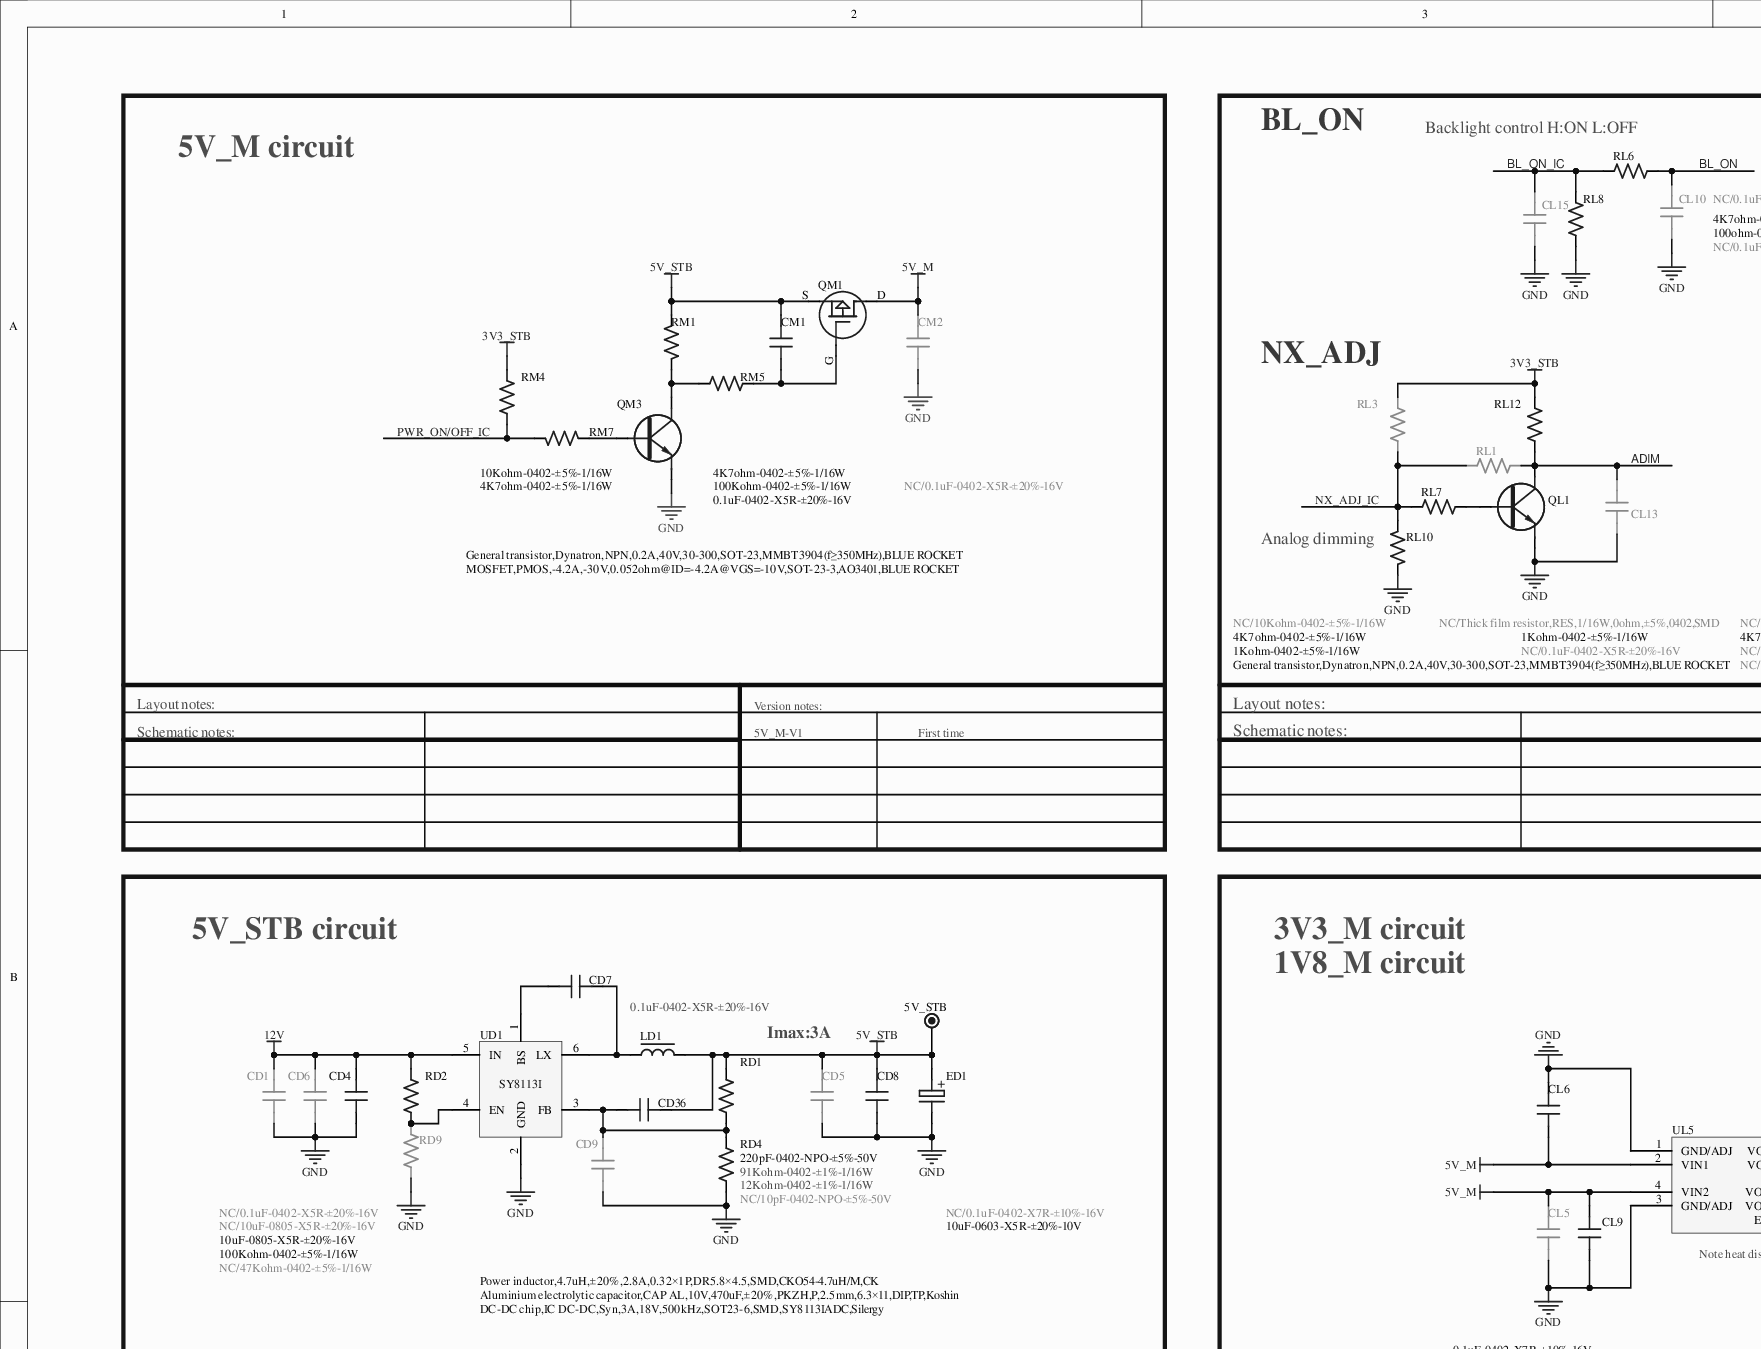
[diagram p0: MISC84395-7.SchDoc, top left]
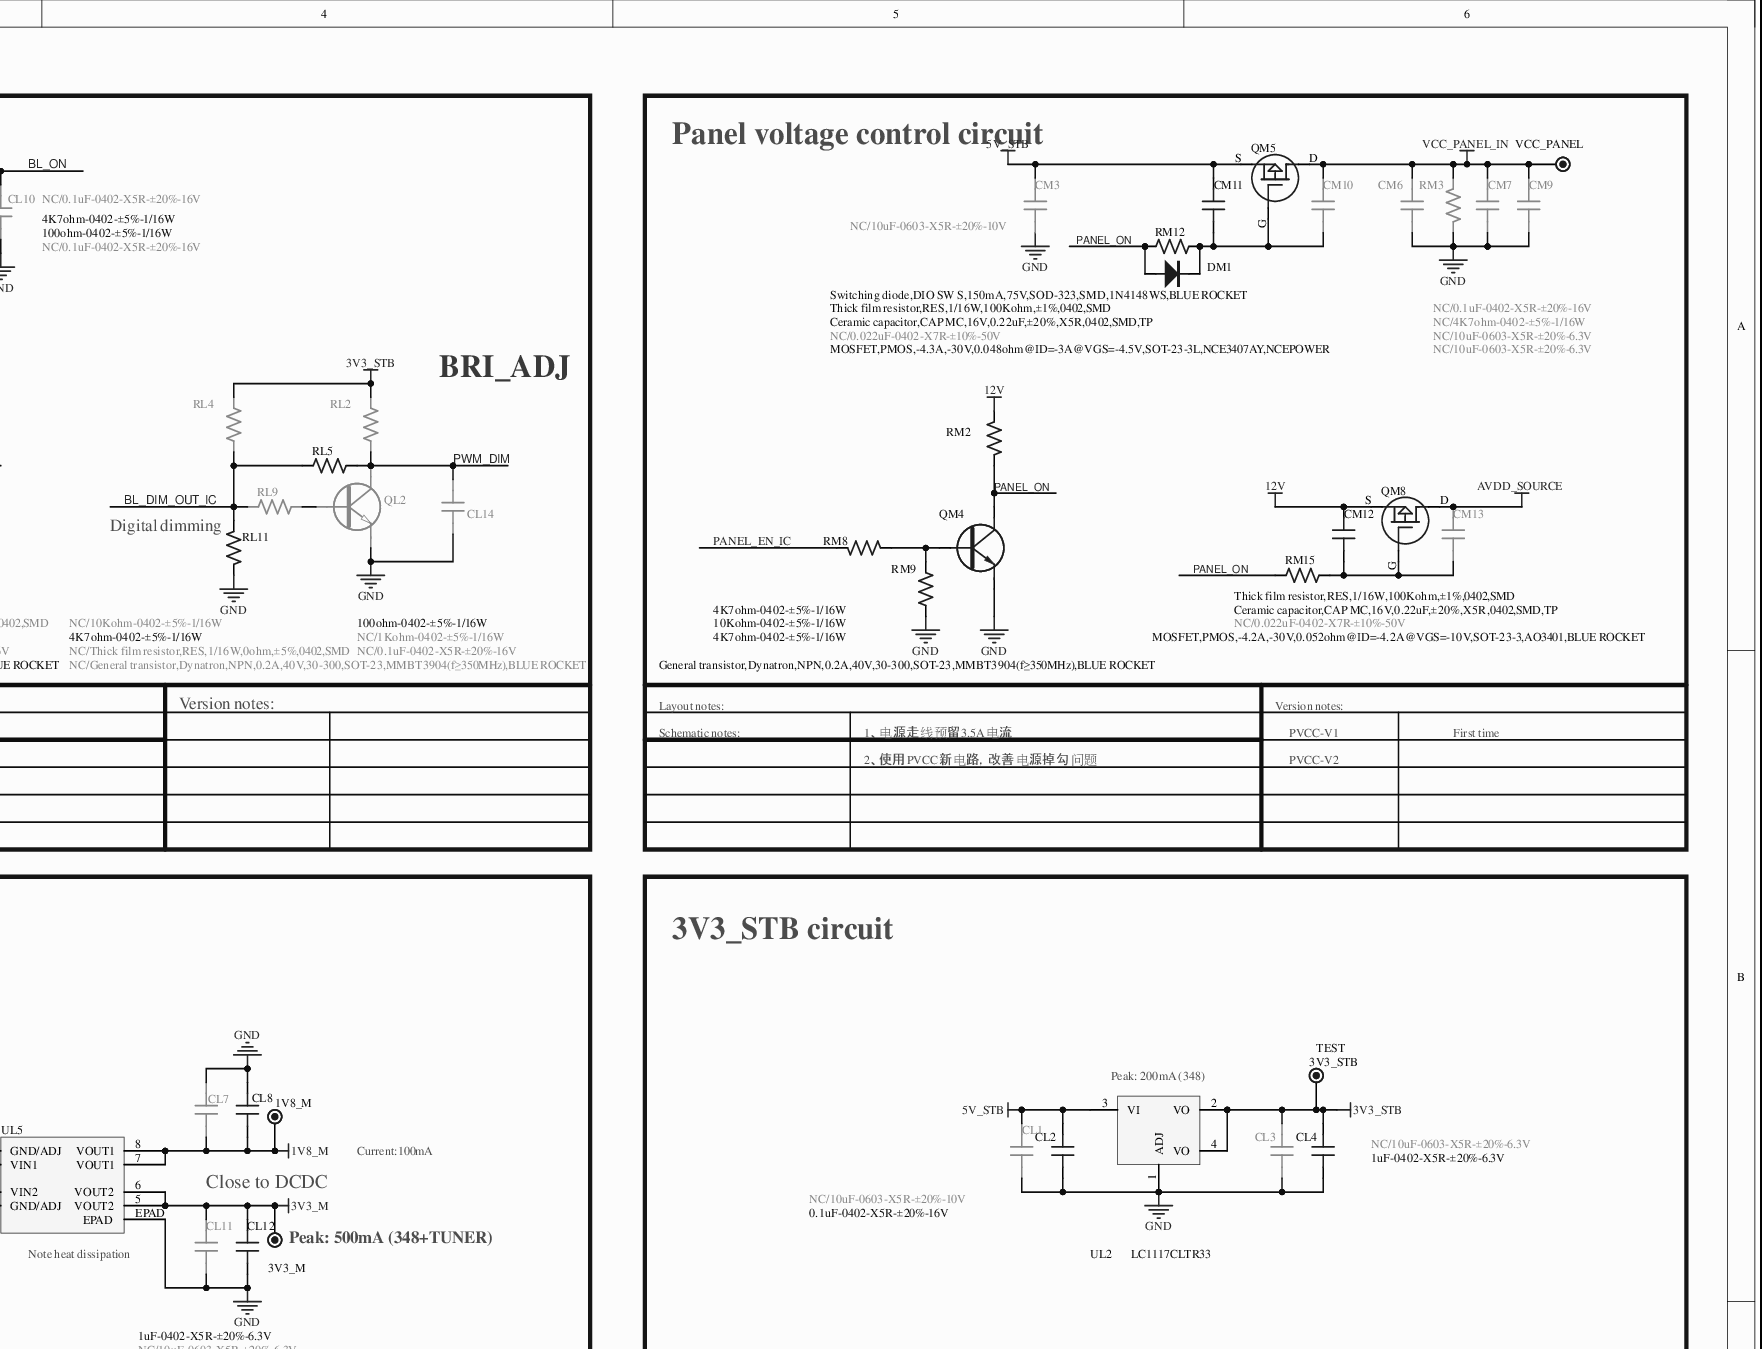
[diagram p1: MISC84395-7.SchDoc, top right]
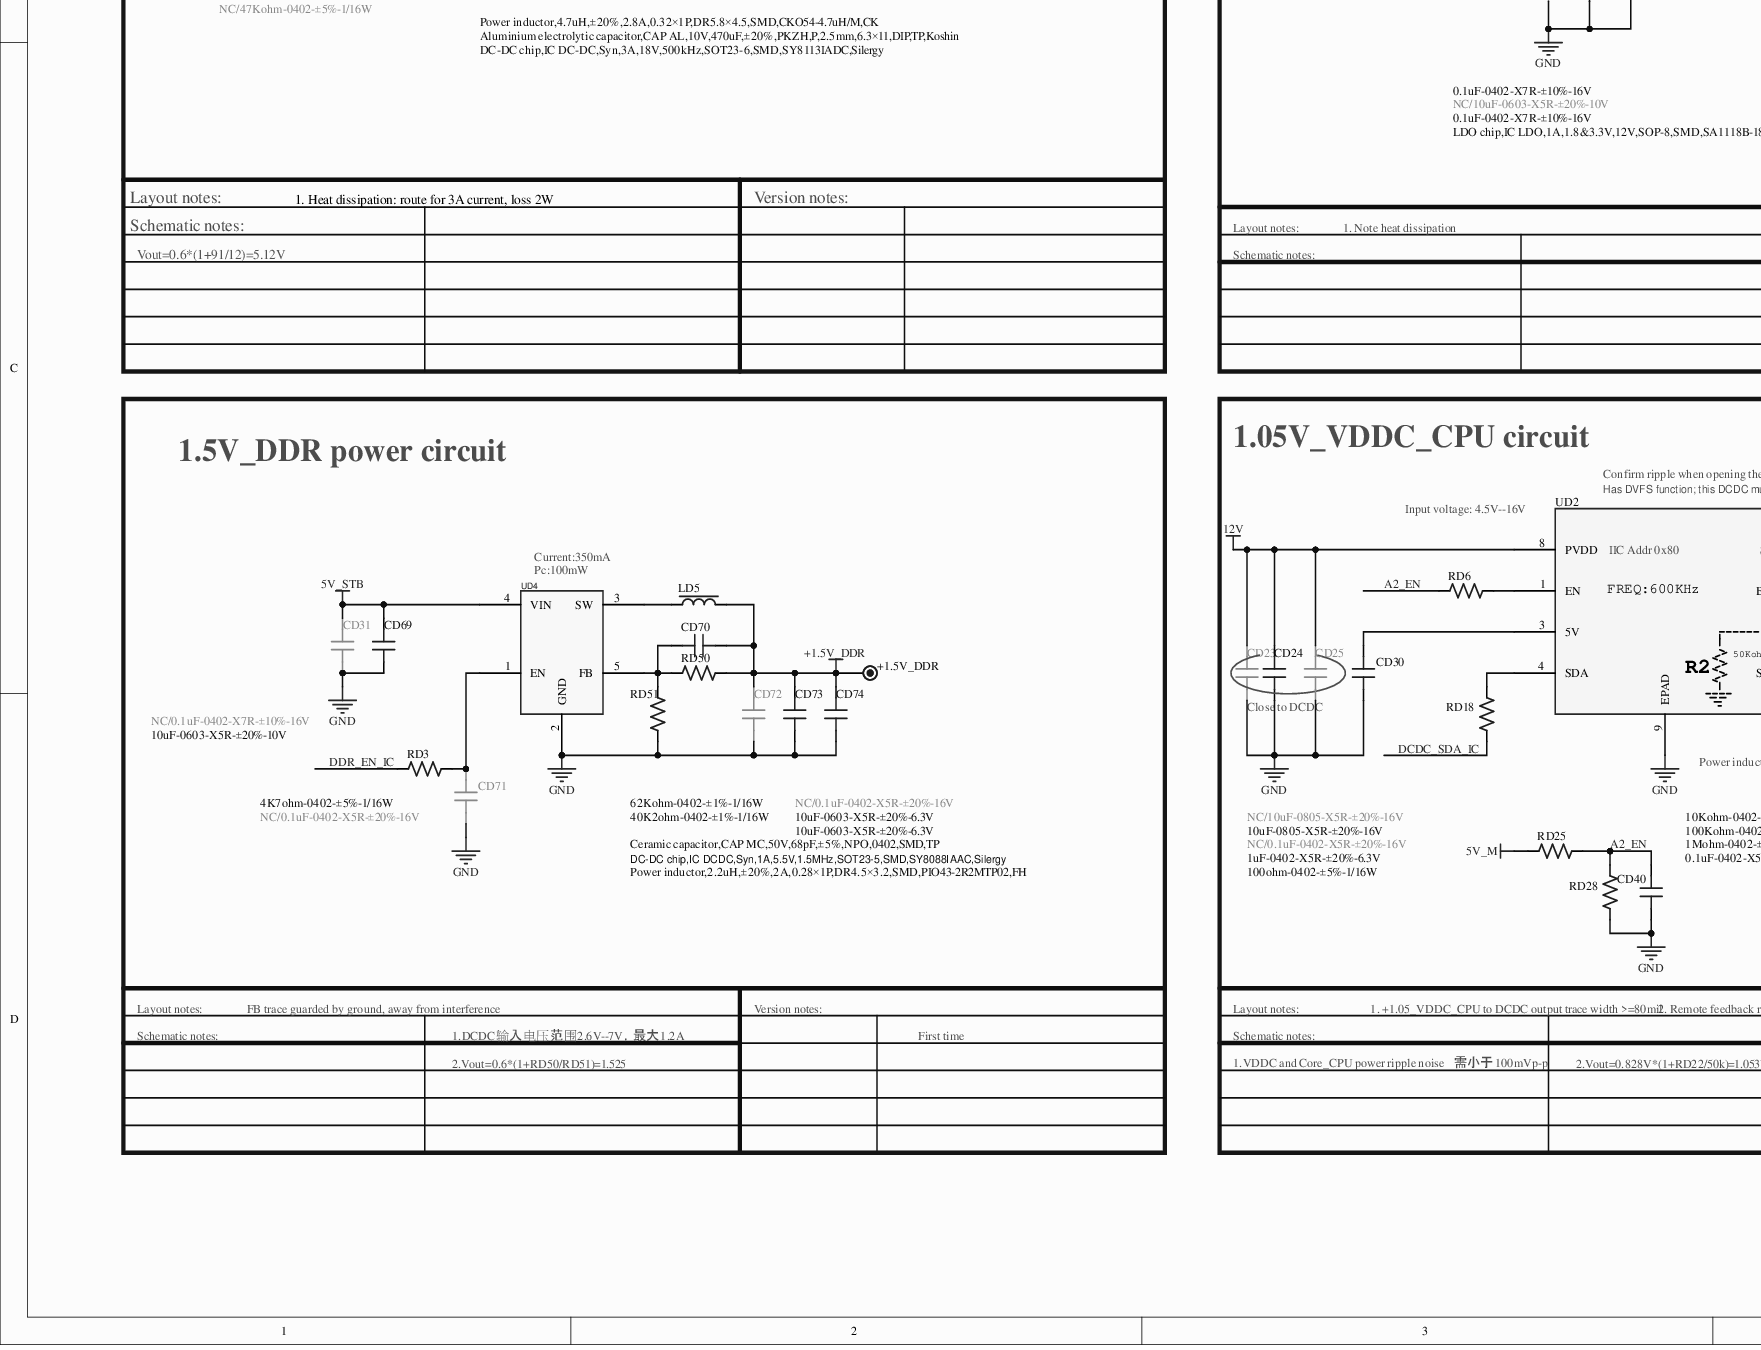
[diagram p2: MISC84395-7.SchDoc, bottom left]
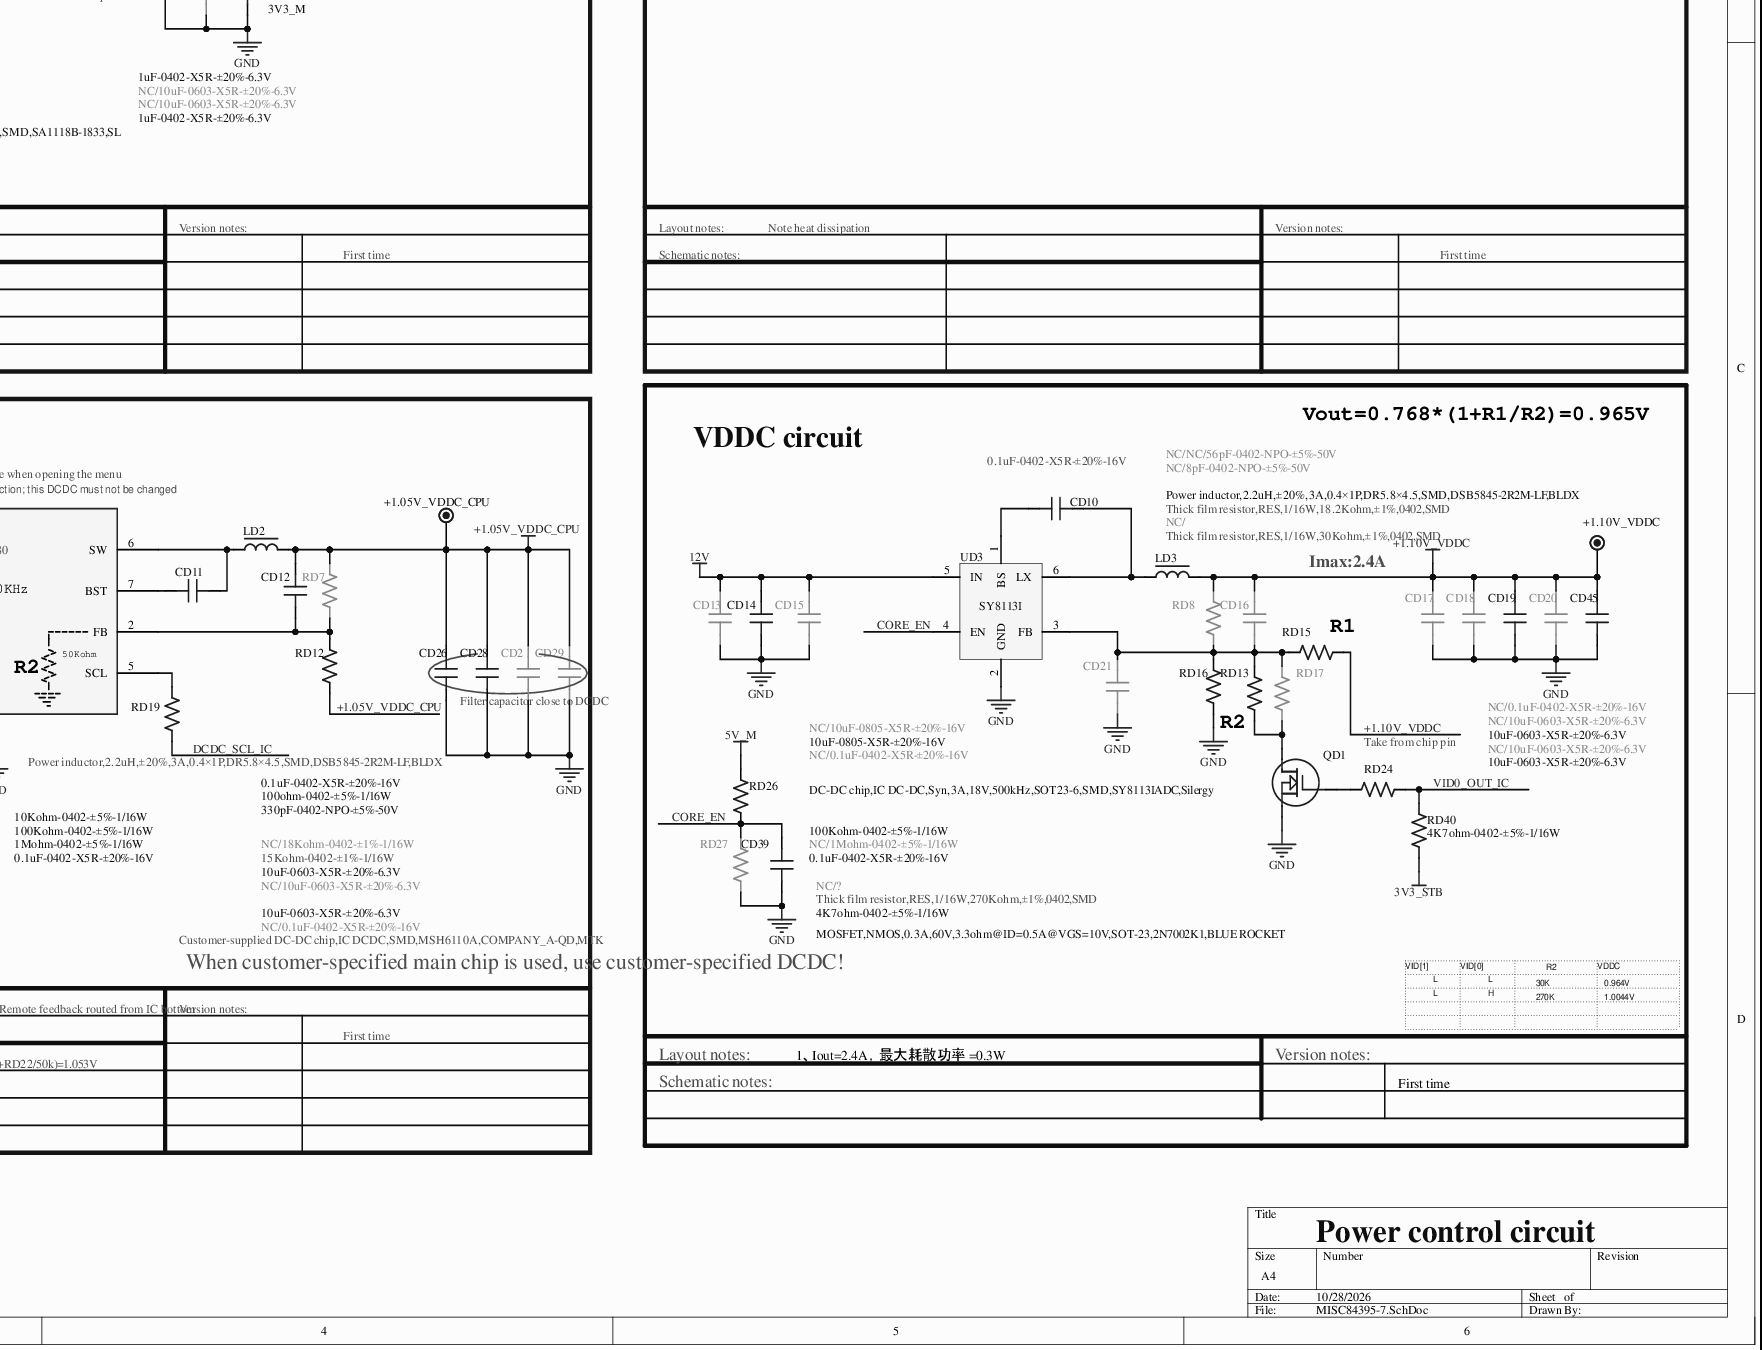
[diagram p3: MISC84395-7.SchDoc, bottom right]
# Altium project MISC84395-37.PrjPCB (part 4 of 13)

## Sheet MISC84395-7.SchDoc
size 635 x 482 mm

### Parts
1V8_M  TEST  [TP]  (value not drawn)
3V3_M  TEST  [TP]  (value not drawn)
3V3_STB  TEST  [TP]
5V_STB  TEST  [TP]  (value not drawn)
+1.5V_DDR  TEST  [TP]  (value not drawn)
+1.05V_VDDC_CPU  TEST  [TP]  (value not drawn)
+1.10V_VDDC  TEST  [TP]  (value not drawn)
CD1  NC/0.1uF-0402-X5R-±20%-16V  [C0402]
CD2  NC/10uF-0603-X5R-±20%-6.3V  [C0603]
CD4  10uF-0805-X5R-±20%-16V  [C0805]
CD5  NC/0.1uF-0402-X7R-±10%-16V  [C0402]
CD6  NC/10uF-0805-X5R-±20%-16V  [C0805]
CD7  0.1uF-0402-X5R-±20%-16V  [C0402]
CD8  10uF-0603-X5R-±20%-10V  [C0603]
CD9  NC/10pF-0402-NPO-±5%-50V  [C0402]
CD10  0.1uF-0402-X5R-±20%-16V  [C0402]
CD11  0.1uF-0402-X5R-±20%-16V  [C0402]
CD12  330pF-0402-NPO-±5%-50V  [C0402]
CD13  NC/10uF-0805-X5R-±20%-16V  [C0805]
CD14  10uF-0805-X5R-±20%-16V  [C0805]
CD15  NC/0.1uF-0402-X5R-±20%-16V  [C0402]
CD16  NC/NC/56pF-0402-NPO-±5%-50V  [C0402]
CD17  NC/0.1uF-0402-X5R-±20%-16V  [C0402]
CD18  NC/10uF-0603-X5R-±20%-6.3V  [C0603]
CD19  10uF-0603-X5R-±20%-6.3V  [C0603]
CD20  NC/10uF-0603-X5R-±20%-6.3V  [C0603]
CD21  NC/8pF-0402-NPO-±5%-50V  [C0402]
CD23  NC/10uF-0805-X5R-±20%-16V  [C0805]
CD24  10uF-0805-X5R-±20%-16V  [C0805]
CD25  NC/0.1uF-0402-X5R-±20%-16V  [C0402]
CD26  10uF-0603-X5R-±20%-6.3V  [C0603]
CD28  10uF-0603-X5R-±20%-6.3V  [C0603]
CD29  NC/0.1uF-0402-X5R-±20%-16V  [C0402]
CD30  1uF-0402-X5R-±20%-6.3V  [C0402]
CD31  NC/0.1uF-0402-X7R-±10%-16V  [C0402]
CD36  220pF-0402-NPO-±5%-50V  [C0402]
CD39  0.1uF-0402-X5R-±20%-16V  [C0402]
CD40  0.1uF-0402-X5R-±20%-16V  [C0402]
CD45  10uF-0603-X5R-±20%-6.3V  [C0603]
CD69  10uF-0603-X5R-±20%-10V  [C0603]
CD70  Ceramic capacitor,CAP MC,50V,68pF,±5%,NPO,0402,SMD,TP  [C0402]
CD71  NC/0.1uF-0402-X5R-±20%-16V  [C0402]
CD72  NC/0.1uF-0402-X5R-±20%-16V  [C0402]
CD73  10uF-0603-X5R-±20%-6.3V  [C0603]
CD74  10uF-0603-X5R-±20%-6.3V  [C0603]
CL1  NC/10uF-0603-X5R-±20%-10V  [C0603]
CL2  0.1uF-0402-X5R-±20%-16V  [C0402]
CL3  NC/10uF-0603-X5R-±20%-6.3V  [C0603]
CL4  1uF-0402-X5R-±20%-6.3V  [C0402]
CL5  NC/10uF-0603-X5R-±20%-10V  [C0603]
CL6  0.1uF-0402-X7R-±10%-16V  [C0402]
CL7  NC/10uF-0603-X5R-±20%-6.3V  [C0603]
CL8  1uF-0402-X5R-±20%-6.3V  [C0402]
CL9  0.1uF-0402-X7R-±10%-16V  [C0402]
CL10  NC/0.1uF-0402-X5R-±20%-16V  [C0402]
CL11  NC/10uF-0603-X5R-±20%-6.3V  [C0603]
CL12  1uF-0402-X5R-±20%-6.3V  [C0402]
CL13  NC/0.1uF-0402-X5R-±20%-16V  [C0402]
CL14  NC/0.1uF-0402-X5R-±20%-16V  [C0402]
CL15  NC/0.1uF-0402-X5R-±20%-16V  [C0402]
CM1  0.1uF-0402-X5R-±20%-16V  [C0402]
CM2  NC/0.1uF-0402-X5R-±20%-16V  [C0402]
CM3  NC/10uF-0603-X5R-±20%-10V  [C0603]
CM6  NC/0.1uF-0402-X5R-±20%-16V  [C0402]
CM7  NC/10uF-0603-X5R-±20%-6.3V  [C0603]
CM9  NC/10uF-0603-X5R-±20%-6.3V  [C0603]
CM10  NC/0.022uF-0402-X7R-±10%-50V  [C0402]
CM11  Ceramic capacitor,CAP MC,16V,0.22uF,±20%,X5R,0402,SMD,TP  [C0402]
CM12  Ceramic capacitor,CAP MC,16V,0.22uF,±20%,X5R,0402,SMD,TP  [C0402]
CM13  NC/0.022uF-0402-X7R-±10%-50V  [C0402]
DM1  Switching diode,DIO SW S,150mA,75V,SOD-323,SMD,1N4148WS,BLUE ROCKET  [DIODE-S-12]
ED1  Aluminium electrolytic capacitor,CAP AL,10V,470uF,±20%,PKZH,P,2.5mm,6.3×11,DIP,TP,Koshin  [EC(6.3*11)-V-2.5]
LD1  Power inductor,4.7uH,±20%,2.8A,0.32×1P,DR5.8×4.5,SMD,CKO54-4.7uH/M,CK  [L(6.0*4.5)-S]
LD2  Power inductor,2.2uH,±20%,3A,0.4×1P,DR5.8×4.5,SMD,DSB5845-2R2M-LF,BLDX  [L(5.8*4.5)-S]
LD3  Power inductor,2.2uH,±20%,3A,0.4×1P,DR5.8×4.5,SMD,DSB5845-2R2M-LF,BLDX  [L(5.8*4.5)-S]
LD5  Power inductor,2.2uH,±20%,2A,0.28×1P,DR4.5×3.2,SMD,PIO43-2R2MTP02,FH  [L(4.5*3.5)-S]
QD1  MOSFET,NMOS,0.3A,60V,3.3ohm@ID=0.5A@VGS=10V,SOT-23,2N7002K1,BLUE ROCKET  [SOT-23-7]
QL1  General transistor,Dynatron,NPN,0.2A,40V,30-300,SOT-23,MMBT3904(f≥350MHz),BLUE ROCKET  [SOT-23]
QL2  NC/General transistor,Dynatron,NPN,0.2A,40V,30-300,SOT-23,MMBT3904(f≥350MHz),BLUE ROCKET  [SOT-23]
QM1  MOSFET,PMOS,-4.2A,-30V,0.052ohm@ID=-4.2A@VGS=-10V,SOT-23-3,AO3401,BLUE ROCKET  [SOT-23-1]
QM3  General transistor,Dynatron,NPN,0.2A,40V,30-300,SOT-23,MMBT3904(f≥350MHz),BLUE ROCKET  [SOT-23]
QM4  General transistor,Dynatron,NPN,0.2A,40V,30-300,SOT-23,MMBT3904(f≥350MHz),BLUE ROCKET  [SOT-23]
QM5  MOSFET,PMOS,-4.3A,-30V,0.048ohm@ID=-3A@VGS=-4.5V,SOT-23-3L,NCE3407AY,NCEPOWER  [SOT-23-1]
QM8  MOSFET,PMOS,-4.2A,-30V,0.052ohm@ID=-4.2A@VGS=-10V,SOT-23-3,AO3401,BLUE ROCKET  [SOT-23-1]
RD1  91Kohm-0402-±1%-1/16W  [R0402]
RD2  100Kohm-0402-±5%-1/16W  [R0402]
RD3  4K7ohm-0402-±5%-1/16W  [R0402]
RD4  12Kohm-0402-±1%-1/16W  [R0402]
RD6  10Kohm-0402-±5%-1/16W  [R0402]
RD7  NC/18Kohm-0402-±1%-1/16W  [R0402]
RD8  NC/  [R0402]
RD9  NC/47Kohm-0402-±5%-1/16W  [R0402]
RD12  15Kohm-0402-±1%-1/16W  [R0402]
RD13  Thick film resistor,RES,1/16W,270Kohm,±1%,0402,SMD  [R0402]
RD15  Thick film resistor,RES,1/16W,18.2Kohm,±1%,0402,SMD  [R0402]
RD16  Thick film resistor,RES,1/16W,30Kohm,±1%,0402,SMD  [R0402]
RD17  NC/?  [R0402]
RD18  100ohm-0402-±5%-1/16W  [R0402]
RD19  100ohm-0402-±5%-1/16W  [R0402]
RD24  4K7ohm-0402-±5%-1/16W  [R0402]
RD25  100Kohm-0402-±5%-1/16W  [R0402]
RD26  100Kohm-0402-±5%-1/16W  [R0402]
RD27  NC/1Mohm-0402-±5%-1/16W  [R0402]
RD28  1Mohm-0402-±5%-1/16W  [R0402]
RD40  4K7ohm-0402-±5%-1/16W  [R0402]
RD50  62Kohm-0402-±1%-1/16W  [R0402]
RD51  40K2ohm-0402-±1%-1/16W  [R0402]
RL1  NC/Thick film resistor,RES,1/16W,0ohm,±5%,0402,SMD  [R0402]
RL2  NC/1Kohm-0402-±5%-1/16W  [R0402]
RL3  NC/10Kohm-0402-±5%-1/16W  [R0402]
RL4  NC/10Kohm-0402-±5%-1/16W  [R0402]
RL5  100ohm-0402-±5%-1/16W  [R0402]
RL6  100ohm-0402-±5%-1/16W  [R0402]
RL7  1Kohm-0402-±5%-1/16W  [R0402]
RL8  4K7ohm-0402-±5%-1/16W  [R0402]
RL9  NC/Thick film resistor,RES,1/16W,0ohm,±5%,0402,SMD  [R0402]
RL10  4K7ohm-0402-±5%-1/16W  [R0402]
RL11  4K7ohm-0402-±5%-1/16W  [R0402]
RL12  1Kohm-0402-±5%-1/16W  [R0402]
RM1  4K7ohm-0402-±5%-1/16W  [R0402]
RM2  4K7ohm-0402-±5%-1/16W  [R0402]
RM3  NC/4K7ohm-0402-±5%-1/16W  [R0402]
RM4  10Kohm-0402-±5%-1/16W  [R0402]
RM5  100Kohm-0402-±5%-1/16W  [R0402]
RM7  4K7ohm-0402-±5%-1/16W  [R0402]
RM8  4K7ohm-0402-±5%-1/16W  [R0402]
RM9  10Kohm-0402-±5%-1/16W  [R0402]
RM12  Thick film resistor,RES,1/16W,100Kohm,±1%,0402,SMD  [R0402]
RM15  Thick film resistor,RES,1/16W,100Kohm,±1%,0402,SMD  [R0402]
UD1  DC-DC chip,IC DC-DC,Syn,3A,18V,500kHz,SOT23-6,SMD,SY8113IADC,Silergy  [TSOT23-6]
UD2  Customer-supplied DC-DC chip,IC DCDC,SMD,MSH6110A,COMPANY_A-QD,MTK  [SOP8/1.27]
UD3  DC-DC chip,IC DC-DC,Syn,3A,18V,500kHz,SOT23-6,SMD,SY8113IADC,Silergy  [TSOT23-6]
UD4  DC-DC chip,IC DCDC,Syn,1A,5.5V,1.5MHz,SOT23-5,SMD,SY8088IAAC,Silergy  [SOT-23-5]
UL2  LC1117CLTR33  [SOT-223]
UL5  LDO chip,IC LDO,1A,1.8&3.3V,12V,SOP-8,SMD,SA1118B-1833,SL  [SOP8/1.27-3]
VCC_PANEL  TEST  [TP]  (value not drawn)

### Blocks framed on the sheet
5V_M circuit: CM1 CM2 QM1 QM3 RM1 RM4 RM5 RM7
Panel voltage control circuit: CM3 CM6 CM7 CM9-CM13 DM1 QM4 QM5 QM8 RM2 RM3 RM8 RM9 RM12 RM15 VCC_PANEL
5V_STB circuit: 5V_STB CD1 CD4-CD9 CD36 ED1 LD1 RD1 RD2 RD4 RD9 UD1
3V3_STB circuit: 3V3_STB CL1-CL4 UL2
VDDC circuit: +1.10V_VDDC CD10 CD13-CD21 CD39 CD45 LD3 QD1 RD8 RD13 RD15-RD17 RD24 RD26 RD27 RD40 UD3
1.5V_DDR power circuit: +1.5V_DDR CD31 CD69-CD74 LD5 RD3 RD50 RD51 UD4
1.05V_VDDC_CPU circuit: +1.05V_VDDC_CPU CD2 CD11 CD12 CD23-CD26 CD28-CD30 CD40 LD2 RD6 RD7 RD12 RD18 RD19 RD25 RD28 UD2

### Nets
1V8_M: 1V8_M.1 CL7.2 CL8.2 UL5.7(VOUT1) UL5.8(VOUT1)
3V3_M: 3V3_M.1 CL11.1 CL12.1 UL5.5(VOUT2) UL5.6(VOUT2)
3V3_STB: 3V3_STB.1 CL3.1 CL4.1 RD40.2 RL2.2 RL3.2 RL4.2 RL12.2 RM4.1 UL2.2(VO) UL2.4(VO)
5V_M: CL5.2 CL6.2 CL9.2 CM2.1 QM1.D RD25.2 RD26.2 UL5.2(VIN1) UL5.4(VIN2)
5V_STB: 5V_STB.1 CD5.1 CD8.2 CD31.2 CD36.2 CD69.2 CL1.2 CL2.1 CM1.1 CM3.2 CM11.2 ED1.1 LD1.2 QM1.S QM5.S RD1.2 RM1.2 UD4.4(VIN) UL2.3(VI)
12V: CD1.2 CD4.1 CD6.1 CD13.1 CD14.1 CD15.1 CD23.2 CD24.2 CD25.2 CM12.2 QM8.S RD2.1 RM2.1 UD1.5(IN) UD2.8(PVDD) UD3.5(IN)
+1.5V_DDR: +1.5V_DDR.1 CD70.2 CD72.2 CD73.1 CD74.1 LD5.2 RD50.2
+1.05V_VDDC_CPU: +1.05V_VDDC_CPU.1 CD2.2 CD12.2 CD26.2 CD28.2 CD29.1 LD2.2 RD7.2 RD12.2
+1.10V_VDDC: +1.10V_VDDC.1 CD16.2 CD17.1 CD18.1 CD19.1 CD20.1 CD45.1 LD3.2 RD8.2 RD15.1
ADIM: CL13.2 QL1.C RL1.2 RL12.1
AVDD_SOURCE: CM13.1 QM8.D
BL_ON: CL10.2 RL6.1
GND: CD1.1 CD2.1 CD4.2 CD5.2 CD6.2 CD8.1 CD9.2 CD13.2 CD14.2 CD15.2 CD17.2 CD18.2 CD19.2 CD20.2 CD21.2 CD23.1 CD24.1 CD25.1 CD26.1 CD28.1 CD29.2 CD30.2 CD31.1 CD39.2 CD40.2 CD45.2 CD69.1 CD71.1 CD72.1 CD73.2 CD74.2 CL1.1 CL2.2 CL3.2 CL4.2 CL5.1 CL6.1 CL7.1 CL8.1 CL9.1 CL10.1 CL11.2 CL12.2 CL13.1 CL14.1 CL15.1 CM2.2 CM3.1 CM6.1 CM7.1 CM9.1 ED1.2 QD1.S QL1.E QL2.E QM3.E QM4.E RD4.1 RD9.1 RD16.1 RD27.2 RD28.2 RD51.1 RL8.1 RL10.2 RL11.2 RM3.2 RM9.2 UD1.2(GND) UD2.9(EPAD) UD3.2(GND) UD4.2(GND) UL2.1(ADJ) UL5.1(GND/ADJ) UL5.3(GND/ADJ) UL5.EPAD
PWM_DIM: CL14.2 QL2.C RL2.1 RL5.1
VCC_PANEL_IN: CM6.2 CM7.2 CM9.2 CM10.1 QM5.D RM3.1 VCC_PANEL.1
A2_EN: CD40.1 RD6.1 RD25.1 RD28.1
BL_DIM_OUT_IC: RL4.1 RL5.2 RL9.2 RL11.1
BL_ON_IC: CL15.2 RL6.2 RL8.2
CORE_EN: CD39.1 RD26.1 RD27.1 UD3.4(EN)
DCDC_SCL_IC: RD19.2
DCDC_SDA_IC: RD18.2
DDR_EN_IC: RD3.2
NX_ADJ_IC: RL1.1 RL3.1 RL7.2 RL10.1
PANEL_EN_IC: RM8.1
PANEL_ON: DM1.A QM4.C RM2.2 RM12.1 RM15.1
PWR_ON/OFF_IC: RM4.2 RM7.1
VID0_OUT_IC: RD24.2 RD40.1
NetCD7_1: CD7.1 UD1.1(BS)
NetCD7_2: CD7.2 LD1.1 UD1.6(LX)
NetCD9_1: CD9.1 CD36.1 RD1.1 RD4.2 UD1.3(FB)
NetCD10_1: CD10.1 UD3.1(BS)
NetCD10_2: CD10.2 LD3.1 UD3.6(LX)
NetCD11_1: CD11.1 LD2.1 UD2.6(SW)
NetCD11_2: CD11.2 UD2.7(BST)
NetCD12_1: CD12.1 RD7.1 RD12.1 UD2.2(FB)
NetCD16_1: CD16.1 CD21.1 RD8.1 RD13.2 RD15.2 RD16.2 RD17.2 UD3.3(FB)
NetCD30_1: CD30.1 UD2.3(5V)
NetCD70_1: CD70.1 RD50.1 RD51.2 UD4.5(FB)
NetCD71_2: CD71.2 RD3.1 UD4.1(EN)
NetCM1_2: CM1.2 QM1.G RM5.2
NetCM10_2: CM10.2 CM11.1 DM1.K QM5.G RM12.2
NetCM12_1: CM12.1 CM13.2 QM8.G RM15.2
NetLD5_1: LD5.1 UD4.3(SW)
NetQD1_D: QD1.D RD13.1 RD17.1
NetQD1_G: QD1.G RD24.1
NetQL1_B: QL1.B RL7.1
NetQL2_B: QL2.B RL9.1
NetQM3_B: QM3.B RM7.2
NetQM3_C: QM3.C RM1.1 RM5.1
NetQM4_B: QM4.B RM8.2 RM9.1
NetRD2_2: RD2.2 RD9.2 UD1.4(EN)
NetRD6_2: RD6.2 UD2.1(EN)
NetRD18_1: RD18.1 UD2.4(SDA)
NetRD19_1: RD19.1 UD2.5(SCL)

### Notes on the sheet
- BL_ON
- (near RL6) Backlight control H:ON L:OFF
- NX_ADJ
- BRI_ADJ
- (near RL10) Analog dimming
- (near RL11) Digital dimming
- Layout notes:
- Version notes:
- Schematic notes:
- 5V_M-V1
- First time
- 1、电源走线预留3.5A电流
- 2、使用PVCC新电路，改善电源掉勾问题
- PVCC-V1
- PVCC-V2
- 3V3_M circuit
- 1V8_M circuit
- Imax:3A
- (near UL2) Peak: 200mA (348)
- Close to DCDC
- Current:100mA
- (near UL5) Note heat dissipation
- (near 3V3_M) Peak: 500mA (348+TUNER)
- 1. Heat dissipation: route for 3A current, loss 2W
- Vout=0.6*(1+91/12)=5.12V
- 1. Note heat dissipation
- Note heat dissipation
- Confirm ripple when opening the menu
- Vout=0.768*(1+R1/R2)=0.965V
- (near UD2) Input voltage: 4.5V--16V
- Has DVFS function; this DCDC must not be changed
- (near UD4) Pc:100mW
- (near UD4) Current:350mA
- Imax:2.4A
- (near RD15) R1
- Filter capacitor close to DCDC
- R2
- Take from chip pin
- FB trace guarded by ground, away from interference
- 1. +1.05_VDDC_CPU to DCDC output trace width >=80mil
- 2. Remote feedback routed from IC bottom
- When customer-specified main chip is used, use customer-specified DCDC!
- VID[1]
- L
- VID[0]
- H
- 30K
- 270K
- VDDC
- 0.964V
- 1.0044V
- 1.DCDC输入电压范围2.6V--7V，最大1.2A
- 2.Vout=0.6*(1+RD50/RD51)=1.525
- 1.VDDC and Core_CPU power ripple noise 需小于100mVp-p
- 2.Vout=0.828V*(1+RD22/50k)=1.053V
- 1、Iout=2.4A，最大耗散功率=0.3W
- Power control circuit

### Library data of the parts
CD1 CD5 CD11 CD15 CD17 CD25 CD29 CD39 CD40 CL2 CL4 CM1 CM2 = 0.1uF-0402-X5R-±20%-16V-D
CD2 CD8 CD26 CD28 CD69 CD73 CD74 CL1 CL3 CL5 CL7 CL11 CM3 CM7 CM9 = 10uF-0603-X5R-±20%-6.3V-D
CD4 CD6 CD13 CD14 CD23 CD24 = 10uF-0805-X5R-±20%-16V-D
CD7 CD10 CD30 = 1uF-0402-X5R-±20%-16V-D
CD9 CD36 = 10pF-0402-NPO-±5%-50V-D
CD12 = 330pF-0402-NPO-±5%-50V-D
CD16 = 56pF-0402-NPO-±5%-50V-D
CD18-CD20 CD45 = 22uF-0603-X5R-±20%-6.3V-D
CD21 = 8pF-0402-NPO-±5%-50V-D
CD31 CL6 CL8 CL9 CL12 = 0.1uF-0402-X7R-±10%-16V-D
CD70 = 004.003.0000573-D: Ceramic capacitor,CAP MC,50V,68pF,±5%,NPO,0402,SMD,TP-D
CD71 CD72 = 0.1uF-0402-X7R-±10%-16V-D: 0.1uF-0402-X5R-±20%-16V
CL10 CL13-CL15 = 0.22uF-0402-X5R-±10%-10V-D
CM6 = 0.1uF-0402-Y5V-+80%-20%-16V-D
CM10 CM13 = 0.022uF-0402-X7R-±10%-50V-D
CM11 CM12 = 004.003.0000398-D: Ceramic capacitor,CAP MC,16V,0.22uF,±20%,X5R,0402,SMD,TP-D
DM1 = 1N4148WS-D
ED1 = 470uF-10V-±20%-6.3×11-105℃-黑底白字-编带-F=2.5-XF-DHAI: Electrolytic
LD1 = SWPA6045S4R7MT-D
LD2 LD3 = SCD54TL-2R2M-D
LD5 = 004.004.0001664-D: Power inductor,2.2uH,±20%,2A,0.28×1P,DR4.5×3.2,SMD,CD43-2.2uH,wenshan-D
QD1 = 2N7002K-7(DIODES)-D
QL1 QL2 QM3 QM4 = KMBT3904-D
QM1 QM5 QM8 = ME2325-G-D: MOS-P
RD1 RD7 RD12 = 18Kohm-0402-±1%-1/16W-D
RD2 RD25 RD26 RM5 = 100Kohm-0402-±5%-1/16W-D
RD3 RD24 RD40 RL2-RL6 RL8 RL12 RM2-RM4 RM8 = 4K7ohm-0402-±5%-1/16W-D
RD4 = 3K3ohm-0402-±1%-1/16W-D
RD6 RM7 RM9 = 10Kohm-0402-±5%-1/16W-D
RD8 = 30Kohm-0402-±1%-1/16W-D
RD9 RD27 RD28 = 1Mohm-0402-±5%-1/16W-D
RD13 = 300Kohm-0402-±1%-1/16W-D
RD15 RD16 = 5K6ohm-0402-±1%-1/16W-D
RD17 = 13Kohm-0402-±1%-1/16W-D
RD18 RD19 = 100ohm-0402-±5%-1/16W-D
RD50 = 62Kohm-0402-±1%-1/16W-D
RD51 = 15Kohm-0402-±1%-1/16W-D
RL1 = 004.002.0000558-D: Thick film resistor,RES,1/16W,0ohm,±5%,0402,SMD-D
RL7 RL9 = 1Kohm-0402-±5%-1/16W-D
RL10 RL11 RM1 = 4k7ohm-0402-±5%-1/16W-D
RM12 RM15 = 004.002.0000578-D: Thick film resistor,RES,1/16W,100Kohm,±1%,0402,SMD-D
UD1 UD3 = 004.010.0001029-D: DC-DC chip,IC DC-DC,Syn,3A,18V,500kHz,SOT23-6,SMD,SY8113IADC,Silergy-D
UD2 = DC-DC芯片,IC DC-DC,Syn,5A,16V,600KHz,ESOP-8,SMD,MSH6110A,Mstar-D
UD4 = DC-DC芯片,IC DCDC,Syn,1.2A,7.0V,1.5MHz,SOT23-5,SMD,LC2127CB5TR,Leadchip-D
UL2 = LC1117CLTR33-D
UL5 = LC1118CS8TR1833-D